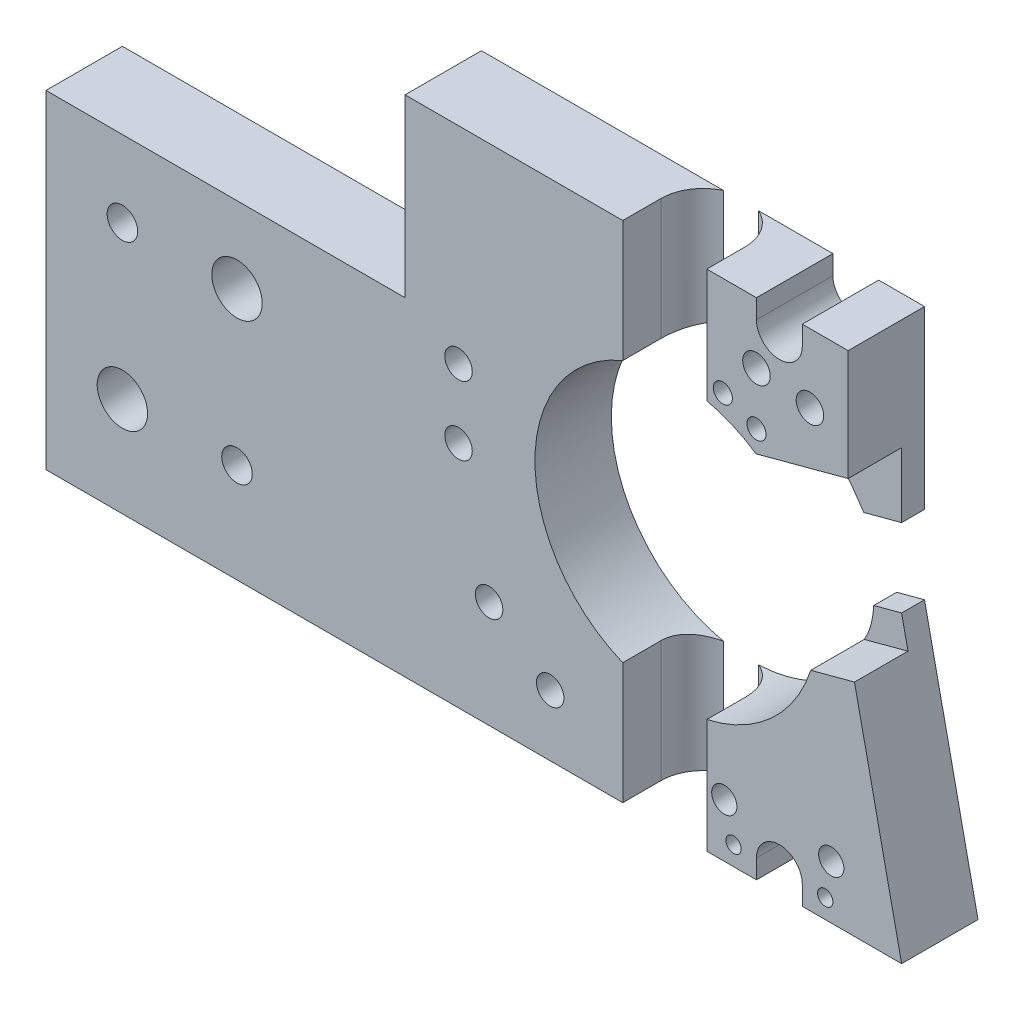
SolidWorks part; units mm, degrees
ref_plane "前视基准面" through (0, 0, 0) normal (0, 0, 1) x (1, 0, 0)
ref_plane "上视基准面" through (0, 0, 0) normal (0, 1, 0) x (1, 0, 0)
ref_plane "右视基准面" through (0, 0, 0) normal (1, 0, 0) x (0, 0, -1)
sketch "草图1" plane through (0, 0, 0) normal (0, 0, 1) x (1, 0, 0)
  line L0 (-50.7639, 4.2656) -> (-3.7639, 4.2656)
  line L1 (-3.7639, 27.2656) -> (54.2361, 27.2656)
  line L2 (-50.7639, 4.2656) -> (-50.7639, -38.7344)
  line L3 (-50.7639, -38.7344) -> (61.2361, -38.7344)
  line L5 (-3.7639, 4.2656) -> (-3.7639, 27.2656)
  line L6 (61.2361, -38.7344) -> (54.2361, -5.9739)
  line L7 (54.2361, -5.9739) -> (50.1886, -7.0584)
  line L8 (54.2361, 27.2656) -> (54.2361, 4.2656)
  line L9 (54.2361, 4.2656) -> (48.2246, 2.6548)
  arc A0 (48.2246, 2.6548) -> (50.1886, -7.0584) centre (31.7361, -5.7344) ccw
  dimension "D5" = 37
  dimension "D1" = 23
  dimension "D2" = 66
  dimension "D3" = 47
  dimension "D4" = 112
  dimension "D7" = 33
  dimension "D9" = 33.5
extrude "凸台-拉伸1" add sketch "草图1" along normal blind 10
sketch "草图2" plane through (0, 27.2656, 0) normal (0, 1, 0) x (1, 0, 0)
  line L0 (35.7361, -5) -> (35.7361, -10)
  line L1 (54.2361, -10) -> (-3.7639, -10) construction
  line L2 (35.7361, -10) -> (24.7361, -10)
  line L3 (24.7361, -10) -> (24.7361, -5)
  line L4 (61.2361, -10) -> (61.2361, 0) construction
  arc A0 (35.7361, -5) -> (24.7361, -5) centre (30.2361, -5) ccw
  dimension "D1" = 5.5
  dimension "D2" = 5
  dimension "D3" = 25.5
extrude "切除-拉伸1" cut sketch "草图2" against normal through all
sketch "草图3" plane through (0, 0, 10) normal (0, 0, 1) x (1, 0, 0)
  line L0 (54.2361, 4.2656) -> (54.2361, 12.7656)
  line L1 (54.2361, 4.2656) -> (54.2361, 27.2656) construction
  line L2 (54.2361, 12.7656) -> (42.1805, 9.5353)
  line L3 (54.2361, -5.9739) -> (55.0719, -9.8856)
  line L4 (61.2361, -38.7344) -> (54.2361, -5.9739) construction
  line L5 (55.0719, -9.8856) -> (49.3403, -11.4214)
  line L6 (54.2361, 4.2656) -> (48.2246, 2.6548)
  line L7 (54.2361, -5.9739) -> (50.1886, -7.0584)
  arc A0 (49.3403, -11.4214) -> (50.1886, -7.0584) centre (31.7361, -5.7344) ccw
  arc A1 (48.2246, 2.6548) -> (42.1805, 9.5353) centre (31.7361, -5.7344) ccw
  dimension "D1" = 4
extrude "切除-拉伸2" cut sketch "草图3" against normal blind 7
sketch "草图4" plane through (0, 0, 10) normal (0, 0, 1) x (1, 0, 0)
  line L0 (42.2361, -36.2344) -> (42.2361, -38.7344)
  line L1 (35.7361, -38.7344) -> (61.2361, -38.7344) construction
  line L2 (48.2361, -36.2344) -> (48.2361, -38.7344)
  line L3 (48.2361, -38.7344) -> (42.2361, -38.7344)
  line L7 (48.2361, 27.2656) -> (42.2361, 27.2656)
  line L8 (42.2361, 24.7656) -> (42.2361, 27.2656)
  line L9 (48.2361, 24.7656) -> (48.2361, 27.2656)
  arc A0 (48.2361, -36.2344) -> (42.2361, -36.2344) centre (45.2361, -36.2344) ccw
  arc A1 (48.2361, 24.7656) -> (42.2361, 24.7656) centre (45.2361, 24.7656) cw
  dimension "D1" = 3
  dimension "D2" = 2.5
  dimension "D3" = 13
extrude "切除-拉伸3" cut sketch "草图4" against normal through all
sketch "草图5" plane through (0, 0, 10) normal (0, 0, 1) x (1, 0, 0)
  line L0 (-3.7639, 4.2656) -> (-50.7639, 4.2656) construction
  line L1 (-50.7639, 4.2656) -> (-50.7639, -38.7344) construction
  line L2 (-50.7639, -38.7344) -> (24.7361, -38.7344) construction
  line L3 (-3.7639, 27.2656) -> (-3.7639, 4.2656) construction
  line L4 (24.7361, 27.2656) -> (-3.7639, 27.2656) construction
  line L6 (24.7361, -38.7344) -> (24.7361, -22.859) construction
  line L7 (35.7361, -38.7344) -> (42.2361, -38.7344) construction
  line L9 (32.5274, -38.7344) -> (32.5274, -24.2175) construction
  line L11 (35.7361, -38.7344) -> (35.7361, -23.7968) construction
  line L12 (48.2361, -38.7344) -> (61.2361, -38.7344) construction
  line L13 (48.2361, -38.7344) -> (48.2361, -36.2344) construction
  line L14 (42.2361, 27.2656) -> (35.7361, 27.2656) construction
  line L15 (54.2361, 12.7656) -> (54.2361, 27.2656) construction
  line L16 (35.7361, 12.328) -> (35.7361, 27.2656) construction
  line L17 (54.2361, 27.2656) -> (48.2361, 27.2656) construction
  line L18 (54.2361, 4.2656) -> (54.2361, 12.7656) construction
  circle A0 centre (-40.7639, -5.7344) radius 2
  circle A1 centre (-40.7639, -25.7344) radius 3.3
  circle A2 centre (-25.7639, -5.7344) radius 3.3
  circle A3 centre (-25.7639, -25.7344) radius 2
  circle A4 centre (7.2361, -24.7344) radius 1.8
  circle A5 centre (15.2361, -30.7344) radius 1.8
  circle A6 centre (3.2361, 0.2656) radius 1.8
  circle A7 centre (3.2361, -8.7344) radius 1.8
  circle A8 centre (38.0274, -31.7344) radius 1.65
  circle A9 centre (52.0261, -31.7344) radius 1.65
  circle A10 centre (42.2361, 19.2656) radius 1.8
  circle A11 centre (49.2361, 18.2656) radius 1.8
  circle A12 centre (37.8361, 14.2656) radius 1.25
  circle A13 centre (42.2361, 12.3856) radius 1.25
  circle A14 centre (39.2361, -36.2344) radius 1
  circle A15 centre (51.2361, -36.2344) radius 1
  dimension "D1" = 4
  dimension "D2" = 6.6
  dimension "D3" = 6.6
  dimension "D4" = 4
  dimension "D13" = 3.6
  dimension "D14" = 3.6
  dimension "D19" = 3.6
  dimension "D20" = 3.6
  dimension "D25" = 3.3
  dimension "D30" = 3.3
  dimension "D33" = 2
  dimension "D34" = 2
  dimension "D37" = 3.6
  dimension "D45" = 2.5
  dimension "D46" = 2.5
  dimension "D48" = 3.6
  dimension "D5" = 10
  dimension "D6" = 10
  dimension "D7" = 15
  dimension "D8" = 10
  dimension "D9" = 13
  dimension "D10" = 10
  dimension "D11" = 15
  dimension "D12" = 13
  dimension "D15" = 7
  dimension "D16" = 27
  dimension "D17" = 9
  dimension "D18" = 7
  dimension "D21" = 14
  dimension "D22" = 17.5
  dimension "D23" = 9.5
  dimension "D24" = 8
  dimension "D26" = 7
  dimension "D27" = 5.5
  dimension "D28" = 2.5
  dimension "D29" = 3.5
  dimension "D31" = 7
  dimension "D32" = 9.21
  dimension "D35" = 2.5
  dimension "D36" = 3
  dimension "D38" = 8
  dimension "D39" = 12
  dimension "D40" = 13
  dimension "D41" = 2.1
  dimension "D42" = 9
  dimension "D43" = 14.88
  dimension "D44" = 12
  dimension "D47" = 5
extrude "切除-拉伸4" cut sketch "草图5" against normal through all
sketch "草图6" plane through (0, 0, 3) normal (0, 0, 1) x (1, 0, 0)
  line L0 (48.2246, 2.6548) -> (54.2361, 4.2656) construction
  line L1 (49.285, 2.9389) -> (48.2246, 2.6548)
  arc A0 (48.2246, 2.6548) -> (42.1805, 9.5353) centre (31.7361, -5.7344) ccw
  spline S0 degree 3 poles (42.1805, 9.5353) (45.5931, 8.5469) (47.48, 5.6494) (49.285, 2.9389) knots 0 0 0 0 1 1 1 1
extrude "切除-拉伸5" cut sketch "草图6" against normal blind 10
sketch "草图7" plane through (0, 0, 3) normal (0, 0, 1) x (1, 0, 0)
  line L0 (54.2361, -5.9739) -> (50.1886, -7.0584) construction
  line L1 (50.5864, -6.9518) -> (50.1886, -7.0584)
  arc A0 (49.3403, -11.4214) -> (50.1886, -7.0584) centre (31.7361, -5.7344) ccw
  spline S0 degree 3 poles (49.3403, -11.4214) (50.1799, -10.066) (50.4746, -8.503) (50.5864, -6.9518) knots 0 0 0 0 1 1 1 1
extrude "切除-拉伸6" cut sketch "草图7" against normal blind 10
